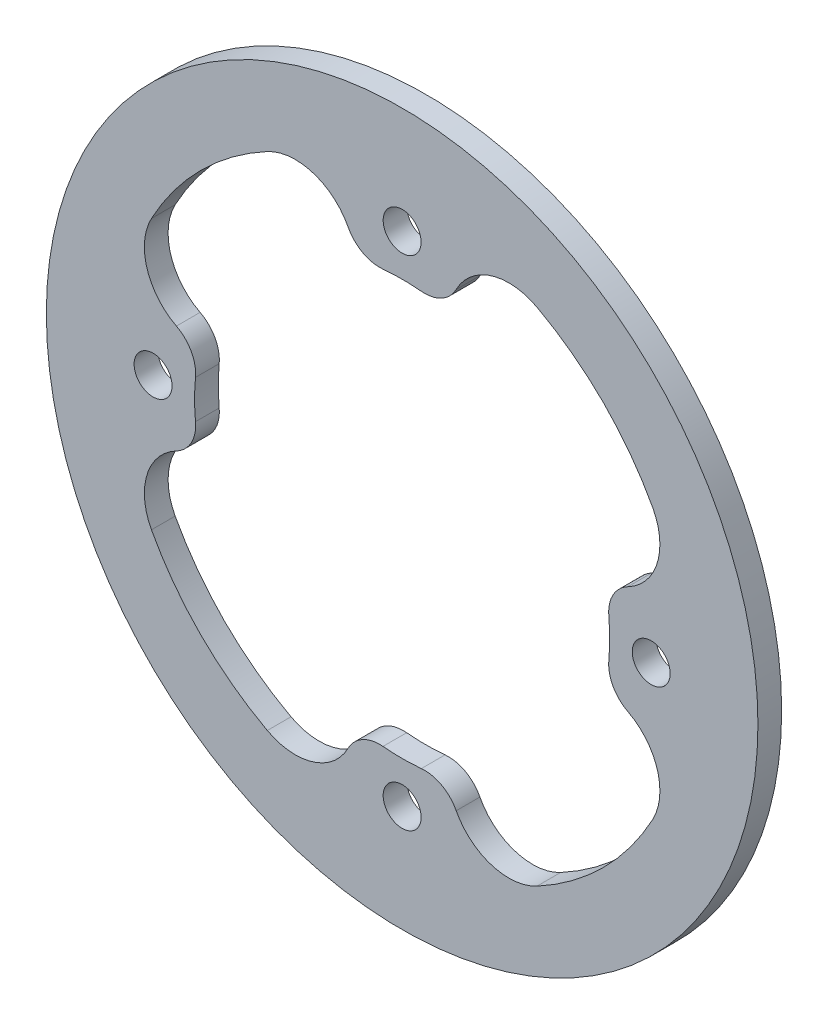
SolidWorks part; units mm, degrees
material "Thornel Mat VMA"
ref_plane "前视基准面" through (0, 0, 0) normal (0, 0, 1) x (1, 0, 0)
ref_plane "上视基准面" through (0, 0, 0) normal (0, 1, 0) x (1, 0, 0)
ref_plane "右视基准面" through (0, 0, 0) normal (1, 0, 0) x (0, 0, -1)
sketch "草图1" plane through (0, 0, 0) normal (0, 0, 1) x (1, 0, 0)
  line L0 (0, 0) -> (24, 0) construction
  line L14 (4, 16.7332) -> (4, 12)
  line L15 (-4, 16.7332) -> (-4, 12)
  line L16 (16.7332, 4) -> (12, 4)
  line L17 (16.7332, -4) -> (12, -4)
  line L18 (4, -16.7332) -> (4, -12)
  line L19 (-4, -16.7332) -> (-4, -12)
  line L20 (-16.7332, -4) -> (-12, -4)
  line L21 (-16.7332, 4) -> (-12, 4)
  circle A0 centre (0, 0) radius 30
  arc A1 (-11.3684, 21.1367) -> (-21.1367, 11.3684) centre (0, 0) ccw
  arc A19 (-6, 8) -> (-8, 6) centre (0, 0) ccw
  arc A33 (4, 12) -> (6, 8) centre (9, 12) ccw
  arc A34 (-4, 12) -> (-6, 8) centre (-9, 12) cw
  arc A35 (4, 16.7332) -> (11.3684, 21.1367) centre (9, 16.7332) cw
  arc A36 (-4, 16.7332) -> (-11.3684, 21.1367) centre (-9, 16.7332) ccw
  arc A37 (16.7332, 4) -> (21.1367, 11.3684) centre (16.7332, 9) ccw
  arc A38 (12, 4) -> (8, 6) centre (12, 9) cw
  arc A39 (16.7332, -4) -> (21.1367, -11.3684) centre (16.7332, -9) cw
  arc A40 (12, -4) -> (8, -6) centre (12, -9) ccw
  arc A41 (4, -16.7332) -> (11.3684, -21.1367) centre (9, -16.7332) ccw
  arc A42 (4, -12) -> (6, -8) centre (9, -12) cw
  arc A43 (-4, -16.7332) -> (-11.3684, -21.1367) centre (-9, -16.7332) cw
  arc A44 (-4, -12) -> (-6, -8) centre (-9, -12) ccw
  arc A45 (-16.7332, -4) -> (-21.1367, -11.3684) centre (-16.7332, -9) ccw
  arc A46 (-12, -4) -> (-8, -6) centre (-12, -9) cw
  arc A47 (-16.7332, 4) -> (-21.1367, 11.3684) centre (-16.7332, 9) cw
  arc A48 (-12, 4) -> (-8, 6) centre (-12, 9) ccw
  arc A49 (-8, -6) -> (-6, -8) centre (0, 0) ccw
  arc A50 (-21.1367, -11.3684) -> (-11.3684, -21.1367) centre (0, 0) ccw
  arc A51 (6, -8) -> (8, -6) centre (0, 0) ccw
  arc A52 (8, 6) -> (6, 8) centre (0, 0) ccw
  arc A53 (11.3684, -21.1367) -> (21.1367, -11.3684) centre (0, 0) ccw
  arc A54 (21.1367, 11.3684) -> (11.3684, 21.1367) centre (0, 0) ccw
  point P15 (0, 0)
  point P40 (0, 0)
  point P51 (0, 0)
  point P94 (0, 0)
  dimension "D1" = 60
  dimension "D2" = 24
  dimension "D5" = 8
  dimension "D6" = 5
  dimension "D8" = 10
  dimension "D7" = 4
extrude "凸台-拉伸1" add sketch "草图1" along normal blind 2
sketch "草图2" plane through (0, 0, 2) normal (0, 0, 1) x (1, 0, 0)
  circle A0 centre (0, 0) radius 21 construction
  circle A1 centre (-21, 0) radius 1.6
  circle A2 centre (0, 21) radius 1.6
  circle A3 centre (21, 0) radius 1.6
  circle A4 centre (0, -21) radius 1.6
  point P14 (0, 0)
  dimension "D1" = 42
  dimension "D2" = 3.2
  dimension "D3" = 4
extrude "切除-拉伸1" cut sketch "草图2" against normal blind 10
sketch "草图3" plane through (0, 0, 2) normal (0, 0, 1) x (1, 0, 0)
  line L0 (0, 6) -> (-6, 0) construction
  line L1 (0, 6) -> (6, 0) construction
  line L2 (-6, 0) -> (0, -6) construction
  line L3 (6, 0) -> (0, -6) construction
  line L4 (-6, 0) -> (6, 0) construction
  line L5 (0, 6) -> (0, -6) construction
  circle A0 centre (0, 6) radius 2.55
  circle A1 centre (-6, 0) radius 2.55
  circle A2 centre (6, 0) radius 2.55
  circle A3 centre (0, -6) radius 2.55
  point P0 (0, 0)
  dimension "D2" = 5.1
  dimension "D1" = 6
extrude "切除-拉伸2" cut sketch "草图3" against normal blind 10
sketch "草图4" plane through (0, 0, 2) normal (0, 0, 1) x (1, 0, 0)
  circle A0 centre (0, 0) radius 17.5
  dimension "D1" = 35
extrude "切除-拉伸3" cut sketch "草图4" against normal blind 10
fillet "圆角1" radius 3 8 edges at (17.0346, -4.0091, 1) (17.0346, 4.0091, 1) (4.0091, -17.0346, 1) (-4.0091, -17.0346, 1) (-17.0346, -4.0091, 1) (-17.0346, 4.0091, 1) (4.0091, 17.0346, 1) (-4.0091, 17.0346, 1)
